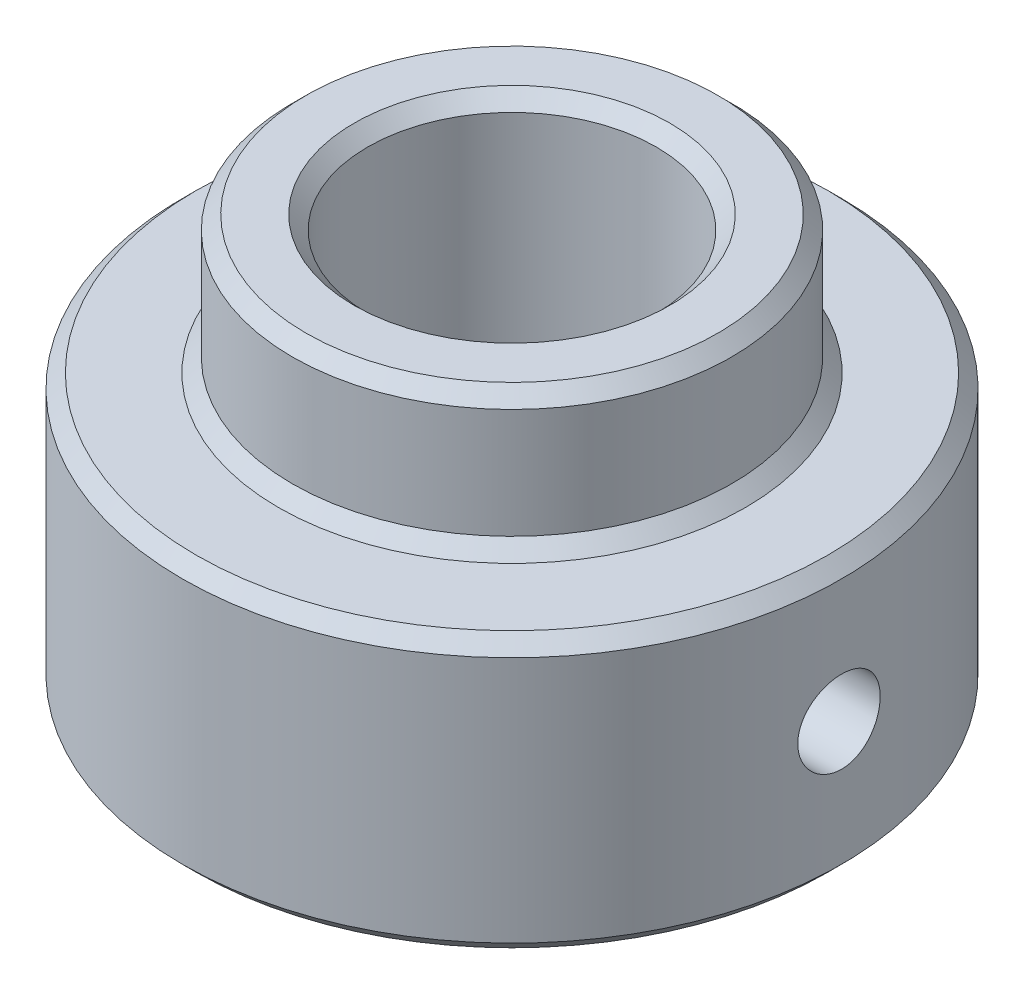
from build123d import *

# Parameters (mm, degrees)
SKETCH1_R               = 24
BOSS_EXTRUDE1_DEPTH     = 20
CUT_EXTRUDE2_DEPTH      = 30
CUT_EXTRUDE2_DEPTH_BACK = 30
SKETCH3_R               = 3
SKETCH4_R               = 16
BOSS_EXTRUDE2_DEPTH     = 10
SKETCH5_R               = 10.5
CUT_EXTRUDE3_DEPTH      = 30
CHAMFER1_SIZE           = 1
CHAMFER2_SIZE           = 1


with BuildPart() as part:
    # Sketch1 → Boss-Extrude1 (new body)
    with BuildSketch(Plane(origin=(0, 0, 0), x_dir=(1, 0, 0), z_dir=(0, 1, 0))):
        with Locations(Location((0, 0, 0), (0, 0, 270))):
            Circle(SKETCH1_R)
    extrude(amount=BOSS_EXTRUDE1_DEPTH)

    # Sketch3 → Cut-Extrude2 (cut, two sides: drawn at the far end of the back side and taken through both)
    with BuildSketch(Plane(origin=(0, 0, 0), x_dir=(0, 0, -1), z_dir=(1, 0, 0)).offset(-CUT_EXTRUDE2_DEPTH_BACK)):
        with Locations(Location((0, 10, 0), (0, 0, 180))):
            Circle(SKETCH3_R)
    extrude(amount=CUT_EXTRUDE2_DEPTH + CUT_EXTRUDE2_DEPTH_BACK, mode=Mode.SUBTRACT)

    # Sketch4 → Boss-Extrude2 (add)
    with BuildSketch(Plane(origin=(0, 20, 0), x_dir=(1, 0, 0), z_dir=(0, 1, 0))):
        with Locations(Location((0, 0, 0), (0, 0, 270))):
            Circle(SKETCH4_R)
    extrude(amount=BOSS_EXTRUDE2_DEPTH)

    # Sketch5 → Cut-Extrude3 (cut)
    with BuildSketch(Plane(origin=(0, 30, 0), x_dir=(1, 0, 0), z_dir=(0, 1, 0))):
        with Locations(Location((0, 0, 0), (0, 0, 270))):
            Circle(SKETCH5_R)
    extrude(amount=-CUT_EXTRUDE3_DEPTH, mode=Mode.SUBTRACT)

    # Chamfer1
    chamfer1_edges = [part.edges().sort_by_distance(p)[0] for p in [
        (0, 20, -16),
        (0, 30, -16),
        (0, 0, -10.5),
        (0, 0, -24),
        (0, 20, -24),
    ]]
    chamfer(chamfer1_edges, length=CHAMFER1_SIZE)

    # Chamfer2
    chamfer2_edges = [part.edges().sort_by_distance(p)[0] for p in [
        (0, 30, -10.5),
    ]]
    chamfer(chamfer2_edges, length=CHAMFER2_SIZE)


solid = part.part
